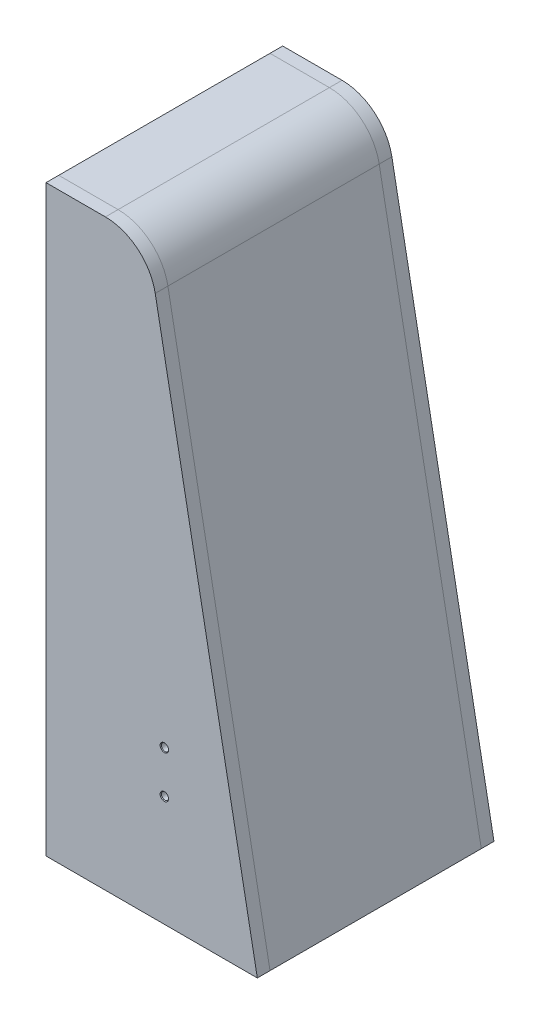
from build123d import *

# Parameters (mm, degrees)
EXTRUDE_1_DEPTH              = 15
EXTRUDE_2_DEPTH              = 250
EXTRUDE_3_DEPTH              = 15
HOLE_WIZARD_M10_1_AT_2_COUNT = 2
HOLE_WIZARD_M10_1_AT_2_PITCH = 50
HOLE_WIZARD_M12_1_AT_2_COUNT = 2
HOLE_WIZARD_M12_1_AT_2_PITCH = 70
HOLE_WIZARD_M12_1_AT_3_COUNT = 2
HOLE_WIZARD_M12_1_AT_3_PITCH = 92.195444573
HOLE_WIZARD_M12_1_AT_4_COUNT = 2
HOLE_WIZARD_M12_1_AT_4_PITCH = 60


with BuildPart() as part:
    # 草图1 → 凸台-拉伸1 (new body)
    with BuildSketch(Plane.XY):
        with BuildLine():
            Line((0, 0), (0, 690))
            Line((0, 690), (70.248731542, 690))
            ThreePointArc((70.248731542, 690), (108.546681021, 676.187304162), (129.211366254, 641.108902192))
            Line((129.211366254, 641.108902192), (250, 0))
            Line((250, 0), (0, 0))
        make_face()
    extrude(amount=EXTRUDE_1_DEPTH)

    # 草图5 → M10 螺纹孔1 (revolve, cut)
    with BuildSketch(Plane(origin=(140, 181, 15), x_dir=(0, -1, 0), z_dir=(1, 0, 0))):
        Polygon((0, 0), (0, 15), (4.25, 15), (4.25, 0.775), (5.025, 0), align=None)
    hole_wizard_m10_1 = revolve(axis=Axis((140, 181, 21.35), (0, 0, -1)), mode=Mode.SUBTRACT)

    # M10 螺纹孔1 at 2: M10 螺纹孔1 ×2
    with Locations(*[(0, -i * HOLE_WIZARD_M10_1_AT_2_PITCH, 0) for i in range(1, HOLE_WIZARD_M10_1_AT_2_COUNT)]):
        add(hole_wizard_m10_1, mode=Mode.SUBTRACT)


with BuildPart() as body_2:
    # 草图2 → 凸台-拉伸2 (new body)
    with BuildSketch(Plane(origin=(0, 0, 0), x_dir=(-1, 0, 0), z_dir=(0, 0, -1))):
        with BuildLine():
            Line((0, 675), (-70.248731542, 675))
            ThreePointArc((-70.248731542, 675), (-98.972193651, 664.640478122), (-114.470707576, 638.331676644))
            Line((-114.470707576, 638.331676644), (-234.736095929, 0))
            Line((-234.736095929, 0), (-250, 0))
            Line((-250, 0), (-129.211366254, 641.108902192))
            ThreePointArc((-129.211366254, 641.108902192), (-108.546681021, 676.187304162), (-70.248731542, 690))
            Line((-70.248731542, 690), (0, 690))
            Line((0, 690), (0, 675))
        make_face()
    extrude(amount=EXTRUDE_2_DEPTH)


with BuildPart() as body_3:
    # 草图3 → 凸台-拉伸3 (new body)
    with BuildSketch(Plane(origin=(0, 0, -250), x_dir=(-1, 0, 0), z_dir=(0, 0, -1))):
        with BuildLine():
            Line((-250, 0), (0, 0))
            Line((0, 0), (0, 690))
            Line((0, 690), (-70.248731542, 690))
            ThreePointArc((-70.248731542, 690), (-108.546681021, 676.187304162), (-129.211366254, 641.108902192))
            Line((-129.211366254, 641.108902192), (-250, 0))
        make_face()
    extrude(amount=EXTRUDE_3_DEPTH)

    # 草图7 → M12 螺纹孔1 (revolve, cut)
    with BuildSketch(Plane(origin=(45, 590, -265), x_dir=(0, 1, 0), z_dir=(1, 0, 0))):
        Polygon((0, 0), (0, 15.001), (5.1, 15.001), (5.1, 0.925), (6.025, 0), align=None)
    hole_wizard_m12_1 = revolve(axis=Axis((45, 590, -271.35), (0, 0, 1)), mode=Mode.SUBTRACT)

    # M12 螺纹孔1 at 2: M12 螺纹孔1 ×2
    with Locations(*[(i * HOLE_WIZARD_M12_1_AT_2_PITCH, 0, 0) for i in range(1, HOLE_WIZARD_M12_1_AT_2_COUNT)]):
        add(hole_wizard_m12_1, mode=Mode.SUBTRACT)

    # M12 螺纹孔1 at 3: M12 螺纹孔1 ×2
    with Locations(*[Vector(0.7592566023652966, -0.6507913734559686, 0) * (i * HOLE_WIZARD_M12_1_AT_3_PITCH) for i in range(1, HOLE_WIZARD_M12_1_AT_3_COUNT)]):
        add(hole_wizard_m12_1, mode=Mode.SUBTRACT)

    # M12 螺纹孔1 at 4: M12 螺纹孔1 ×2
    with Locations(*[(0, -i * HOLE_WIZARD_M12_1_AT_4_PITCH, 0) for i in range(1, HOLE_WIZARD_M12_1_AT_4_COUNT)]):
        add(hole_wizard_m12_1, mode=Mode.SUBTRACT)


solid = Compound([part.part, body_2.part, body_3.part])
